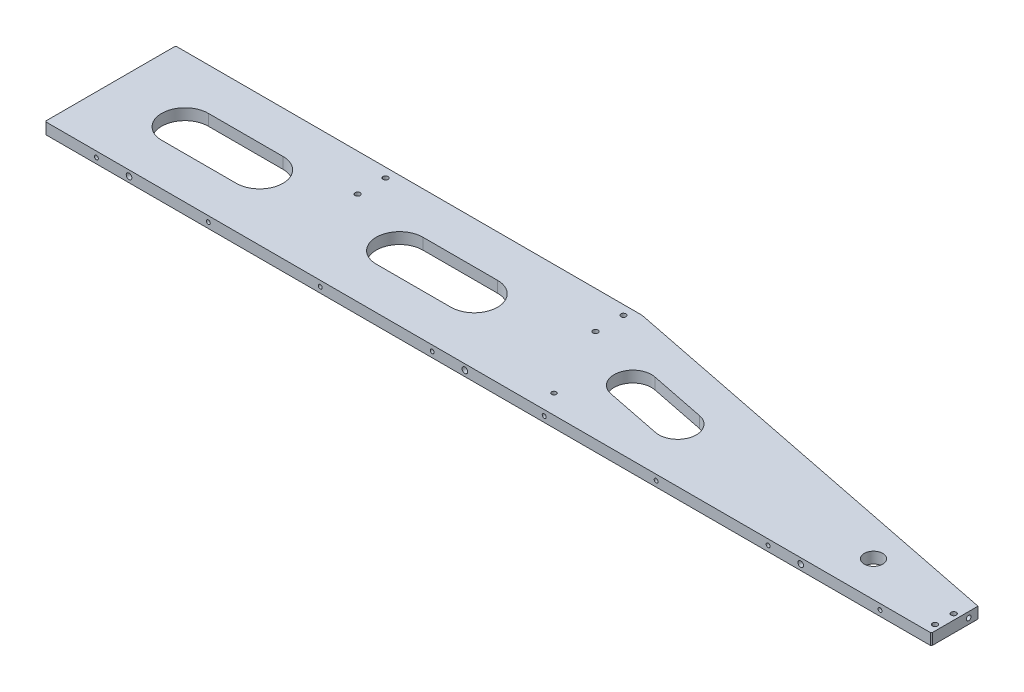
from build123d import *

# Parameters (mm, degrees)
BOSS_EXTRUDE2_DEPTH                              = 12
SKETCH9_R                                        = 10
CUT_EXTRUDE3_DEPTH                               = 12
M4_TAPPED_HOLE2_D                                = 3.3
M4_TAPPED_HOLE2_DEPTH                            = 10.1
M4_TAPPED_HOLE2_TIP                              = 0.991420021
M6_TAPPED_HOLE1_D                                = 5
M6_TAPPED_HOLE1_DEPTH                            = 15
M6_TAPPED_HOLE1_TIP                              = 1.502151548
M4_TAPPED_HOLE3_D                                = 3.3
M4_TAPPED_HOLE3_DEPTH                            = 11.5
M4_TAPPED_HOLE3_TIP                              = 0.991420021
M4_TAPPED_HOLE4_D                                = 3.3
M4_TAPPED_HOLE4_DEPTH                            = 11.5
M4_TAPPED_HOLE4_TIP                              = 0.991420021
M6_TAPPED_HOLE3_D                                = 5
M6_TAPPED_HOLE3_DEPTH                            = 17
M6_TAPPED_HOLE3_TIP                              = 1.502151548
M6_TAPPED_HOLE2_D                                = 5
M6_TAPPED_HOLE2_DEPTH                            = 23
M6_TAPPED_HOLE2_TIP                              = 1.502151548
F_6_0_6_DIAMETER_HOLE1_D                         = 6
F_6_0_6_DIAMETER_HOLE1_DEPTH                     = 15
F_6_0_6_DIAMETER_HOLE1_TIP                       = 1.802581857
M5_TAPPED_HOLE1_D                                = 4.2
M5_TAPPED_HOLE1_DEPTH                            = 12.4
M5_TAPPED_HOLE1_TIP                              = 1.2618073
F_6_0_6_DIAMETER_HOLE2_D                         = 6
F_6_0_6_DIAMETER_HOLE2_DEPTH                     = 15
F_6_0_6_DIAMETER_HOLE2_TIP                       = 1.802581857
HOLE_SIZE_PER_HEX_SOCKET_SCREW_TYPE1_D           = 5.5
HOLE_SIZE_PER_HEX_SOCKET_SCREW_TYPE1_CBORE_D     = 10
HOLE_SIZE_PER_HEX_SOCKET_SCREW_TYPE1_CBORE_DEPTH = 5.7
CHAMFER2_SIZE                                    = 1


with BuildPart() as part:
    # Sketch2 → Boss-Extrude2 (new body)
    with BuildSketch(Plane(origin=(0, 0, 0), x_dir=(-1, 0, 0), z_dir=(0, -1, 0))):
        Polygon((0, 0), (0, 140), (-500, 140), (-950, 50), (-950, 0), align=None)
    extrude(amount=-BOSS_EXTRUDE2_DEPTH)

    # Sketch9 → Cut-Extrude3 (cut)
    with BuildSketch(Plane.XZ):
        with Locations((850, -38)):
            Circle(SKETCH9_R)
        with BuildLine():
            Line((80, -45), (160, -45))
            ThreePointArc((160, -45), (185, -70), (160, -95))
            Line((160, -95), (80, -95))
            ThreePointArc((80, -95), (55, -70), (80, -45))
        make_face()
        with BuildLine():
            Line((310, -45), (390, -45))
            ThreePointArc((390, -45), (415, -70), (390, -95))
            Line((390, -95), (310, -95))
            ThreePointArc((310, -95), (285, -70), (310, -45))
        make_face()
        with BuildLine():
            Line((556.077677297, -50.388386486), (616.077677297, -38.388386486))
            ThreePointArc((616.077677297, -38.388386486), (639.611613514, -54.077677297), (623.922322703, -77.611613514))
            Line((623.922322703, -77.611613514), (563.922322703, -89.611613514))
            ThreePointArc((563.922322703, -89.611613514), (540.388386486, -73.922322703), (556.077677297, -50.388386486))
        make_face()
    extrude(amount=-CUT_EXTRUDE3_DEPTH, mode=Mode.SUBTRACT)

    # M4 Tapped Hole2
    with Locations(Plane(origin=(0, 0, 0), x_dir=(-1, 0, 0), z_dir=(0, -1, 0))):
        with Locations((-275, 10), (-275, 30), (-795, 23), (-905, 23), (-795, 53), (-905, 53)):
            Hole(M4_TAPPED_HOLE2_D / 2, depth=M4_TAPPED_HOLE2_DEPTH)
            with Locations((0, 0, -(M4_TAPPED_HOLE2_DEPTH + M4_TAPPED_HOLE2_TIP / 2))):  # 118° drill point
                Cone(0, M4_TAPPED_HOLE2_D / 2, M4_TAPPED_HOLE2_TIP, mode=Mode.SUBTRACT)

    # M6 Tapped Hole1
    with Locations(Plane(origin=(0, 0, 0), x_dir=(-1, 0, 0), z_dir=(0, -1, 0))):
        with Locations((-525, 20.5)):
            Hole(M6_TAPPED_HOLE1_D / 2, depth=M6_TAPPED_HOLE1_DEPTH)
            with Locations((0, 0, -(M6_TAPPED_HOLE1_DEPTH + M6_TAPPED_HOLE1_TIP / 2))):  # 118° drill point
                Cone(0, M6_TAPPED_HOLE1_D / 2, M6_TAPPED_HOLE1_TIP, mode=Mode.SUBTRACT)

    # M4 Tapped Hole3
    with Locations(Plane(origin=(0, 0, -140), x_dir=(-1, 0, 0), z_dir=(0, 0, -1))):
        with Locations((-50, 6), (-400, 6)):
            Hole(M4_TAPPED_HOLE3_D / 2, depth=M4_TAPPED_HOLE3_DEPTH)
            with Locations((0, 0, -(M4_TAPPED_HOLE3_DEPTH + M4_TAPPED_HOLE3_TIP / 2))):  # 118° drill point
                Cone(0, M4_TAPPED_HOLE3_D / 2, M4_TAPPED_HOLE3_TIP, mode=Mode.SUBTRACT)

    # M4 Tapped Hole4
    with Locations(Plane(origin=(46.153846154, 0, -230.769230769), x_dir=(-0.9805806756909201, 0, -0.19611613513818424), z_dir=(0.19611613513818424, 0, -0.9805806756909201))):
        with Locations((-871.745835149, 6), (-521.745835149, 6)):
            Hole(M4_TAPPED_HOLE4_D / 2, depth=M4_TAPPED_HOLE4_DEPTH)
            with Locations((0, 0, -(M4_TAPPED_HOLE4_DEPTH + M4_TAPPED_HOLE4_TIP / 2))):  # 118° drill point
                Cone(0, M4_TAPPED_HOLE4_D / 2, M4_TAPPED_HOLE4_TIP, mode=Mode.SUBTRACT)

    # M6 Tapped Hole3
    with Locations(Plane(origin=(950, 0, 0), x_dir=(0, 0, -1), z_dir=(1, 0, 0))):
        with Locations((40, 6), (40, 96)):
            Hole(M6_TAPPED_HOLE3_D / 2, depth=M6_TAPPED_HOLE3_DEPTH)
            with Locations((0, 0, -(M6_TAPPED_HOLE3_DEPTH + M6_TAPPED_HOLE3_TIP / 2))):  # 118° drill point
                Cone(0, M6_TAPPED_HOLE3_D / 2, M6_TAPPED_HOLE3_TIP, mode=Mode.SUBTRACT)

    # M6 Tapped Hole2
    with Locations(Plane.ZY):
        with Locations((-15, 6), (-70, 6), (-125, 6)):
            Hole(M6_TAPPED_HOLE2_D / 2, depth=M6_TAPPED_HOLE2_DEPTH)
            with Locations((0, 0, -(M6_TAPPED_HOLE2_DEPTH + M6_TAPPED_HOLE2_TIP / 2))):  # 118° drill point
                Cone(0, M6_TAPPED_HOLE2_D / 2, M6_TAPPED_HOLE2_TIP, mode=Mode.SUBTRACT)

    # Ø6.0 (6) Diameter Hole1
    with Locations(Plane.ZY):
        with Locations((-30, 6), (-110, 6)):
            Hole(F_6_0_6_DIAMETER_HOLE1_D / 2, depth=F_6_0_6_DIAMETER_HOLE1_DEPTH)
            with Locations((0, 0, -(F_6_0_6_DIAMETER_HOLE1_DEPTH + F_6_0_6_DIAMETER_HOLE1_TIP / 2))):  # 118° drill point
                Cone(0, F_6_0_6_DIAMETER_HOLE1_D / 2, F_6_0_6_DIAMETER_HOLE1_TIP, mode=Mode.SUBTRACT)

    # M5 Tapped Hole1
    with Locations(Plane.XY):
        with Locations((55, 6), (175, 6), (295, 6), (415, 6), (535, 6), (655, 6), (775, 6), (895, 6)):
            Hole(M5_TAPPED_HOLE1_D / 2, depth=M5_TAPPED_HOLE1_DEPTH)
            with Locations((0, 0, -(M5_TAPPED_HOLE1_DEPTH + M5_TAPPED_HOLE1_TIP / 2))):  # 118° drill point
                Cone(0, M5_TAPPED_HOLE1_D / 2, M5_TAPPED_HOLE1_TIP, mode=Mode.SUBTRACT)

    # Ø6.0 (6) Diameter Hole2
    with Locations(Plane.XY):
        with Locations((90, 6), (450, 6), (810, 6)):
            Hole(F_6_0_6_DIAMETER_HOLE2_D / 2, depth=F_6_0_6_DIAMETER_HOLE2_DEPTH)
            with Locations((0, 0, -(F_6_0_6_DIAMETER_HOLE2_DEPTH + F_6_0_6_DIAMETER_HOLE2_TIP / 2))):  # 118° drill point
                Cone(0, F_6_0_6_DIAMETER_HOLE2_D / 2, F_6_0_6_DIAMETER_HOLE2_TIP, mode=Mode.SUBTRACT)

    # Hole size per hex socket screw type1 (through all)
    with Locations(Plane(origin=(0, 0, 0), x_dir=(-1, 0, 0), z_dir=(0, -1, 0))):
        with Locations((-235, 100), (-235, 130), (-490, 100), (-490, 130), (-944, 10), (-944, 30)):
            CounterBoreHole(HOLE_SIZE_PER_HEX_SOCKET_SCREW_TYPE1_D / 2, HOLE_SIZE_PER_HEX_SOCKET_SCREW_TYPE1_CBORE_D / 2, HOLE_SIZE_PER_HEX_SOCKET_SCREW_TYPE1_CBORE_DEPTH)

    # Chamfer2
    chamfer2_edges = [part.edges().sort_by_distance(p)[0] for p in [
        (950, 6, 0),
        (0, 6, -140),
        (0, 6, 0),
    ]]
    chamfer(chamfer2_edges, length=CHAMFER2_SIZE)


solid = part.part
